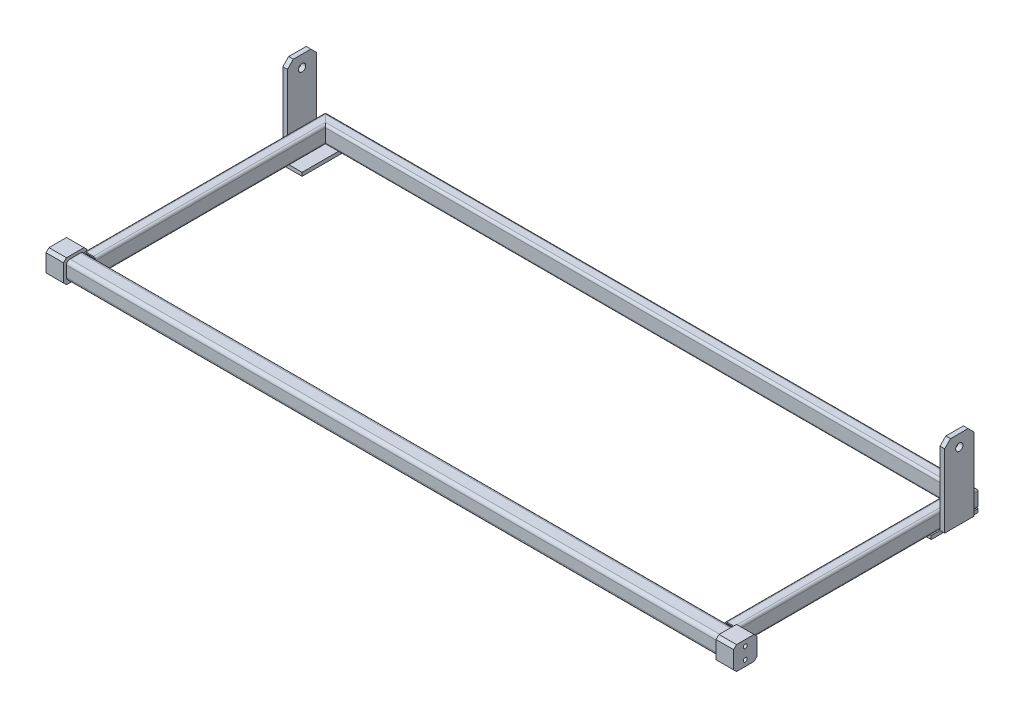
from build123d import *

# Parameters (mm, degrees)
COLD_FORMED_HOLLOW_SQUARE_STEEL_GB_T_67_DEPTH = 1116
COLD_FORMED_HOLLOW_RECTANGULAR_STEEL_GB_DEPTH = 422.027756377
COLD_FORMED_HOLLOW_RECTANGULAR_STEEL_3_DEPTH  = 1134.055512755
COLD_FORMED_HOLLOW_RECTANGULAR_STEEL_5_DEPTH  = 422.027756377
BOSS_EXTRUDE1_DEPTH                           = 30
SKETCH5_R                                     = 1.70107459
CUT_EXTRUDE1_DEPTH                            = 30
M8_TAPPED_HOLE1_AT_2_COUNT                    = 2
M8_TAPPED_HOLE1_AT_2_PITCH                    = 20
SKETCH7_W                                     = 40
SKETCH7_H                                     = 80
BOSS_EXTRUDE2_DEPTH                           = 6
BOSS_EXTRUDE2_2_DEPTH                         = 6
SKETCH9_R                                     = 6.25
BOSS_EXTRUDE3_DEPTH                           = 8
SKETCH10_R                                    = 2
CUT_EXTRUDE2_DEPTH                            = 8
M6_TAPPED_HOLE1_AT_2_COUNT                    = 2
M6_TAPPED_HOLE1_AT_2_PITCH                    = 35
M6_TAPPED_HOLE1_AT_3_COUNT                    = 2
M6_TAPPED_HOLE1_AT_3_PITCH                    = 70
M6_TAPPED_HOLE1_AT_4_COUNT                    = 2
M6_TAPPED_HOLE1_AT_4_PITCH                    = 105


with BuildPart() as part:
    # Sketch11 → Cold-formed hollow square steel (GB/T 6728-2002) 30×3(1) (new body)
    with BuildSketch(Plane(origin=(0, 0, 0), x_dir=(0, 0, -1), z_dir=(1, 0, 0))):
        with BuildLine():
            Line((-9, -15), (9, -15))
            ThreePointArc((9, -15), (13.242640687, -13.242640687), (15, -9))
            Line((15, -9), (15, 9))
            ThreePointArc((15, 9), (13.242640687, 13.242640687), (9, 15))
            Line((9, 15), (-9, 15))
            ThreePointArc((-9, 15), (-13.242640687, 13.242640687), (-15, 9))
            Line((-15, 9), (-15, -9))
            ThreePointArc((-15, -9), (-13.242640687, -13.242640687), (-9, -15))
        make_face()
        with BuildLine():
            Line((-9, -12), (9, -12))
            ThreePointArc((9, -12), (11.121320344, -11.121320344), (12, -9))
            Line((12, -9), (12, 9))
            ThreePointArc((12, 9), (11.121320344, 11.121320344), (9, 12))
            Line((9, 12), (-9, 12))
            ThreePointArc((-9, 12), (-11.121320344, 11.121320344), (-12, 9))
            Line((-12, 9), (-12, -9))
            ThreePointArc((-12, -9), (-11.121320344, -11.121320344), (-9, -12))
        make_face(mode=Mode.SUBTRACT)
    extrude(amount=COLD_FORMED_HOLLOW_SQUARE_STEEL_GB_T_67_DEPTH)


with BuildPart() as body_2:
    # Sketch1 → Cold-formed hollow rectangular steel (GB/T 6728-2002) 30×20×2(1) (new body)
    with BuildSketch(Plane(origin=(1106, 0, -15), x_dir=(1, 0, 0), z_dir=(0, 0, -1))):
        with BuildLine():
            Line((-6, -15), (6, -15))
            ThreePointArc((6, -15), (8.828427125, -13.828427125), (10, -11))
            Line((10, -11), (10, 11))
            ThreePointArc((10, 11), (8.828427125, 13.828427125), (6, 15))
            Line((6, 15), (-6, 15))
            ThreePointArc((-6, 15), (-8.828427125, 13.828427125), (-10, 11))
            Line((-10, 11), (-10, -11))
            ThreePointArc((-10, -11), (-8.828427125, -13.828427125), (-6, -15))
        make_face()
        with BuildLine():
            Line((-6, -13), (6, -13))
            ThreePointArc((6, -13), (7.414213562, -12.414213562), (8, -11))
            Line((8, -11), (8, 11))
            ThreePointArc((8, 11), (7.414213562, 12.414213562), (6, 13))
            Line((6, 13), (-6, 13))
            ThreePointArc((-6, 13), (-7.414213562, 12.414213562), (-8, 11))
            Line((-8, 11), (-8, -11))
            ThreePointArc((-8, -11), (-7.414213562, -12.414213562), (-6, -13))
        make_face(mode=Mode.SUBTRACT)
    extrude(amount=COLD_FORMED_HOLLOW_RECTANGULAR_STEEL_GB_DEPTH)

    # Cold-formed hollow rectangular steel 2
    split(bisect_by=Plane(origin=(1106, 0, -418), x_dir=(0, 1, 0), z_dir=(0.707106781, 0, 0.707106781)), keep=Keep.TOP)


with BuildPart() as body_3:
    # Sketch1 on segment 2 (carried to segment 2) → Cold-formed hollow rectangular steel 3 (new body)
    with BuildSketch(Plane(origin=(1125.027756377, 0, -418), x_dir=(0, 0, -1), z_dir=(-1, 0, 0))):
        with BuildLine():
            Line((-6, -15), (6, -15))
            ThreePointArc((6, -15), (8.828427125, -13.828427125), (10, -11))
            Line((10, -11), (10, 11))
            ThreePointArc((10, 11), (8.828427125, 13.828427125), (6, 15))
            Line((6, 15), (-6, 15))
            ThreePointArc((-6, 15), (-8.828427125, 13.828427125), (-10, 11))
            Line((-10, 11), (-10, -11))
            ThreePointArc((-10, -11), (-8.828427125, -13.828427125), (-6, -15))
        make_face()
        with BuildLine():
            Line((-6, -13), (6, -13))
            ThreePointArc((6, -13), (7.414213562, -12.414213562), (8, -11))
            Line((8, -11), (8, 11))
            ThreePointArc((8, 11), (7.414213562, 12.414213562), (6, 13))
            Line((6, 13), (-6, 13))
            ThreePointArc((-6, 13), (-7.414213562, 12.414213562), (-8, 11))
            Line((-8, 11), (-8, -11))
            ThreePointArc((-8, -11), (-7.414213562, -12.414213562), (-6, -13))
        make_face(mode=Mode.SUBTRACT)
    extrude(amount=COLD_FORMED_HOLLOW_RECTANGULAR_STEEL_3_DEPTH)

    # Cold-formed hollow rectangular steel 3 m
    split(bisect_by=Plane(origin=(10, 0, -418), x_dir=(0, 1, 0), z_dir=(0.707106781, 0, -0.707106781)), keep=Keep.TOP)

    # Cold-formed hollow rectangular steel 4
    split(bisect_by=Plane(origin=(1106, 0, -418), x_dir=(0, -1, 0), z_dir=(-0.707106781, 0, -0.707106781)), keep=Keep.TOP)

    # Sketch10 → Cut-Extrude2 (cut)
    with BuildSketch(Plane(origin=(0, 0, -428), x_dir=(-1, 0, 0), z_dir=(0, 0, -1))):
        with Locations(Location((-776, 0, 0), (0, 0, 90))):
            Circle(SKETCH10_R)
        with Locations(Location((-741, 0, 0), (0, 0, 90))):
            Circle(SKETCH10_R)
        with Locations(Location((-706, 0, 0), (0, 0, 90))):
            Circle(SKETCH10_R)
        with Locations(Location((-671, 0, 0), (0, 0, 90))):
            Circle(SKETCH10_R)
    extrude(amount=-CUT_EXTRUDE2_DEPTH, mode=Mode.SUBTRACT)

    # 草图11 → M6 Tapped Hole1 (revolve, cut)
    with BuildSketch(Plane(origin=(671, 0, -428), x_dir=(0, 1, 0), z_dir=(1, 0, 0))):
        Polygon((0, 0), (0, 18.502151548), (2.5, 17), (2.5, 0), align=None)
    m6_tapped_hole1 = revolve(axis=Axis((671, 0, -434.35), (0, 0, 1)), mode=Mode.SUBTRACT)

    # M6 Tapped Hole1 at 2: M6 Tapped Hole1 ×2
    with Locations(*[(i * M6_TAPPED_HOLE1_AT_2_PITCH, 0, 0) for i in range(1, M6_TAPPED_HOLE1_AT_2_COUNT)]):
        add(m6_tapped_hole1, mode=Mode.SUBTRACT)

    # M6 Tapped Hole1 at 3: M6 Tapped Hole1 ×2
    with Locations(*[(i * M6_TAPPED_HOLE1_AT_3_PITCH, 0, 0) for i in range(1, M6_TAPPED_HOLE1_AT_3_COUNT)]):
        add(m6_tapped_hole1, mode=Mode.SUBTRACT)

    # M6 Tapped Hole1 at 4: M6 Tapped Hole1 ×2
    with Locations(*[(i * M6_TAPPED_HOLE1_AT_4_PITCH, 0, 0) for i in range(1, M6_TAPPED_HOLE1_AT_4_COUNT)]):
        add(m6_tapped_hole1, mode=Mode.SUBTRACT)


with BuildPart() as body_4:
    # Sketch1 on segment 3 (carried to segment 3) → Cold-formed hollow rectangular steel 5 (new body)
    with BuildSketch(Plane(origin=(10, 0, -437.027756377), x_dir=(-1, 0, 0), z_dir=(0, 0, 1))):
        with BuildLine():
            Line((-6, -15), (6, -15))
            ThreePointArc((6, -15), (8.828427125, -13.828427125), (10, -11))
            Line((10, -11), (10, 11))
            ThreePointArc((10, 11), (8.828427125, 13.828427125), (6, 15))
            Line((6, 15), (-6, 15))
            ThreePointArc((-6, 15), (-8.828427125, 13.828427125), (-10, 11))
            Line((-10, 11), (-10, -11))
            ThreePointArc((-10, -11), (-8.828427125, -13.828427125), (-6, -15))
        make_face()
        with BuildLine():
            Line((-6, -13), (6, -13))
            ThreePointArc((6, -13), (7.414213562, -12.414213562), (8, -11))
            Line((8, -11), (8, 11))
            ThreePointArc((8, 11), (7.414213562, 12.414213562), (6, 13))
            Line((6, 13), (-6, 13))
            ThreePointArc((-6, 13), (-7.414213562, 12.414213562), (-8, 11))
            Line((-8, 11), (-8, -11))
            ThreePointArc((-8, -11), (-7.414213562, -12.414213562), (-6, -13))
        make_face(mode=Mode.SUBTRACT)
    extrude(amount=COLD_FORMED_HOLLOW_RECTANGULAR_STEEL_5_DEPTH)

    # Cold-formed hollow rectangular steel 5 m
    split(bisect_by=Plane(origin=(10, 0, -418), x_dir=(0, -1, 0), z_dir=(-0.707106781, 0, 0.707106781)), keep=Keep.TOP)


with BuildPart() as body_5:
    # Sketch4 → Boss-Extrude1 (new body)
    with BuildSketch(Plane.ZY):
        Polygon((-20, 15), (-15, 20), (15, 20), (20, 15), (20, -15), (15, -20), (-15, -20), (-20, -15), align=None)
    boss_extrude1 = extrude(amount=BOSS_EXTRUDE1_DEPTH)

    # Sketch5 → Cut-Extrude1 (cut)
    with BuildSketch(Plane.ZY.offset(30)):
        with Locations((0, 10)):
            Circle(SKETCH5_R)
        with Locations((0, -10)):
            Circle(SKETCH5_R)
    cut_extrude1 = extrude(amount=-CUT_EXTRUDE1_DEPTH, mode=Mode.SUBTRACT)


with BuildPart() as m8_tapped_hole1_tool:
    # Sketch6 → M8 Tapped Hole1 (revolve)
    with BuildSketch(Plane(origin=(-30, 10, 0), x_dir=(0, 0, 1), z_dir=(0, 1, 0))):
        Polygon((0, 0), (0, 32.042926105), (3.4, 30), (3.4, 0), align=None)
    m8_tapped_hole1 = revolve(axis=Axis((-36.35, 10, 0), (1, 0, 0)))


with BuildPart() as part_1:
    add(part.part)

    # M8 Tapped Hole1: cut by m8_tapped_hole1_tool
    add(m8_tapped_hole1_tool.part, mode=Mode.SUBTRACT)


with BuildPart() as body_5_1:
    add(body_5.part)

    # M8 Tapped Hole1: cut by m8_tapped_hole1_tool
    add(m8_tapped_hole1_tool.part, mode=Mode.SUBTRACT)


with BuildPart() as m8_tapped_hole1_at_2_tool:
    # M8 Tapped Hole1 at 2: M8 Tapped Hole1 ×2
    with Locations(*[(0, -i * M8_TAPPED_HOLE1_AT_2_PITCH, 0) for i in range(1, M8_TAPPED_HOLE1_AT_2_COUNT)]):
        add(m8_tapped_hole1)


with BuildPart() as part_2:
    add(part_1.part)

    # M8 Tapped Hole1 at 2: cut by m8_tapped_hole1_at_2_tool
    add(m8_tapped_hole1_at_2_tool.part, mode=Mode.SUBTRACT)


with BuildPart() as body_5_2:
    add(body_5_1.part)

    # M8 Tapped Hole1 at 2: cut by m8_tapped_hole1_at_2_tool
    add(m8_tapped_hole1_at_2_tool.part, mode=Mode.SUBTRACT)


with BuildPart() as body_6:
    # Sketch7 → Boss-Extrude2 (new body)
    with BuildSketch(Plane.XZ.offset(15)):
        with Locations((1096, -388)):
            Rectangle(SKETCH7_W, SKETCH7_H)
    extrude(amount=BOSS_EXTRUDE2_DEPTH)


with BuildPart() as body_7:
    # Sketch7 → Boss-Extrude2 2 (new body)
    with BuildSketch(Plane.XZ.offset(15)):
        with Locations((20, -388)):
            Rectangle(SKETCH7_W, SKETCH7_H)
    extrude(amount=BOSS_EXTRUDE2_2_DEPTH)


with BuildPart() as body_8:
    # Sketch9 → Boss-Extrude3 (new body)
    with BuildSketch(Plane.ZY):
        Polygon((-413, -15), (-363, -15), (-363, 110), (-373, 120), (-403, 120), (-413, 110), align=None)
        with Locations((-388, 100)):
            Circle(SKETCH9_R, mode=Mode.SUBTRACT)
    boss_extrude3 = extrude(amount=BOSS_EXTRUDE3_DEPTH)


with BuildPart() as part_3:
    add(part_2.part)

    add(body_2.part)  # Mirror1 merges body 2
    # Mirror1: Boss-Extrude1, Cut-Extrude1, M8 Tapped Hole1, Boss-Extrude3 across plane
    add(boss_extrude1.mirror(Plane.ZY.offset(-558)))
    add(cut_extrude1.mirror(Plane.ZY.offset(-558)), mode=Mode.SUBTRACT)
    add(m8_tapped_hole1.mirror(Plane.ZY.offset(-558)), mode=Mode.SUBTRACT)
    add(boss_extrude3.mirror(Plane.ZY.offset(-558)))

    # Mirror1 copy 1 sketch → Mirror1 copy 1 (revolve, cut)
    with BuildSketch(Plane(origin=(1146, -10, 0), x_dir=(0, 0, 1), z_dir=(0, 1, 0))):
        Polygon((0, 0), (0, -32.042926105), (3.4, -30), (3.4, 0), align=None)
    revolve(axis=Axis((1152.35, -10, 0), (1, 0, 0)), mode=Mode.SUBTRACT)


solid = Compound([body_3.part, body_4.part, body_5_2.part, body_6.part, body_7.part, body_8.part, part_3.part])
